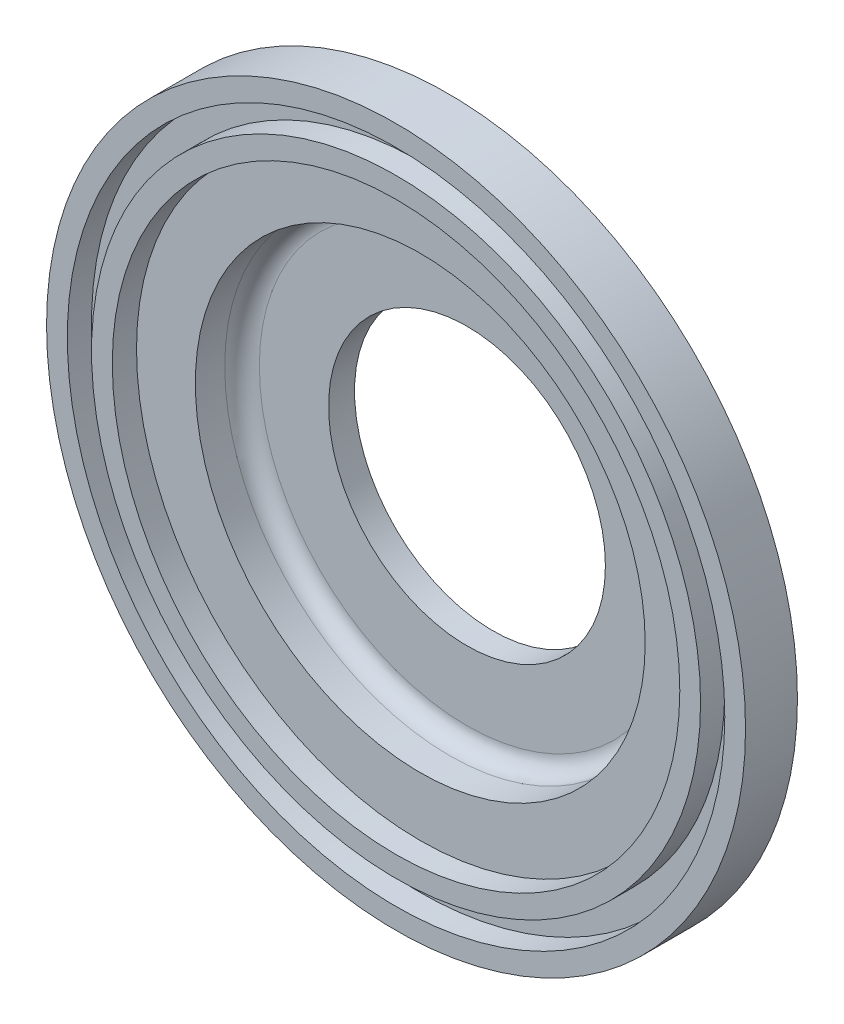
from build123d import *

# Parameters (mm, degrees)
FILLET1_R = 10


with BuildPart() as part:
    # Sketch1 → Revolve1 (revolve)
    with BuildSketch(Plane(origin=(0, 0, 0), x_dir=(0, 0, -1), z_dir=(1, 0, 0)), mode=Mode.PRIVATE) as revolve1_sk:
        Polygon((0, 164), (0, 176), (14, 176), (14, 190), (0, 190), (0, 202), (30, 202), (30, 145), (56, 145), (56, 80), (41, 80), (41, 130), (14, 130), (14, 164), align=None)
    revolve(revolve1_sk.sketch.rotate(Axis((0, 0, 0), (0, 0, -1)), 90), axis=Axis((0, 0, 0), (0, 0, -1)))

    # Fillet1
    fillet1_edges = [part.edges().sort_by_distance(p)[0] for p in [
        (-130, 0, -41),
    ]]
    fillet(fillet1_edges, radius=FILLET1_R)


solid = part.part
